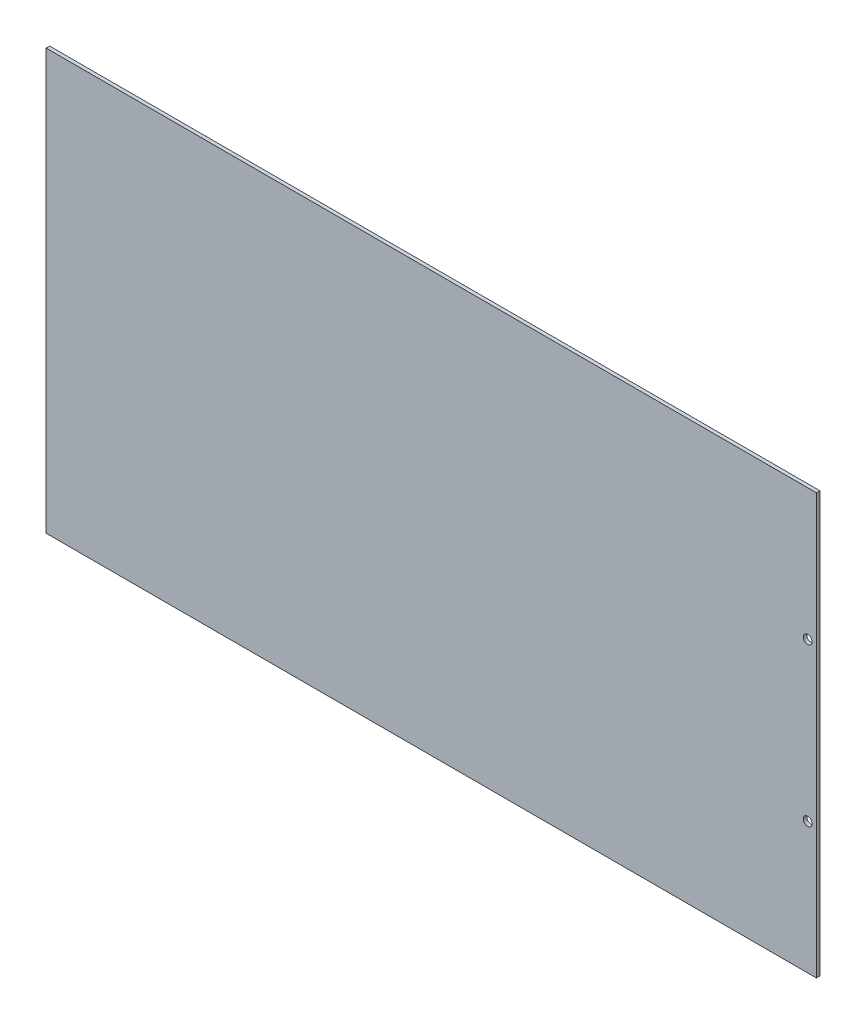
SolidWorks part; units mm, degrees
ref_plane "前视基准面" through (0, 0, 0) normal (0, 0, 1) x (1, 0, 0)
ref_plane "上视基准面" through (0, 0, 0) normal (0, 1, 0) x (1, 0, 0)
ref_plane "右视基准面" through (0, 0, 0) normal (1, 0, 0) x (0, 0, -1)
sketch "草图1" plane through (0, 0, 0) normal (0, 0, 1) x (1, 0, 0)
  line L1 (-220, 120) -> (220, 120)
  line L2 (-220, 120) -> (-220, -120)
  line L3 (-220, -120) -> (220, -120)
  line L4 (220, 120) -> (220, -120)
  line L5 (-220, 120) -> (220, -120) construction
  line L6 (-220, -120) -> (220, 120) construction
  point P0 (0, 0)
  dimension "D1" = 240
  dimension "D2" = 440
extrude "凸台-拉伸1" add sketch "草图1" along normal blind 2
sketch "草图2" plane through (0, 0, 2) normal (0, 0, 1) x (1, 0, 0)
  line L0 (244.4977, 59.9966) -> (204.4977, 59.9966) construction
  line L1 (220, -120) -> (220, 120) construction
  line L2 (244.4977, -30.0034) -> (204.4977, -30.0034) construction
  circle A0 centre (215, 44.9966) radius 2.5
  circle A1 centre (215, -45.0034) radius 2.5
  dimension "D3" = 5
  dimension "D4" = 5
  dimension "D1" = 15
  dimension "D2" = 5
  dimension "D5" = 15
extrude "切除-拉伸1" cut sketch "草图2" against normal blind 2
